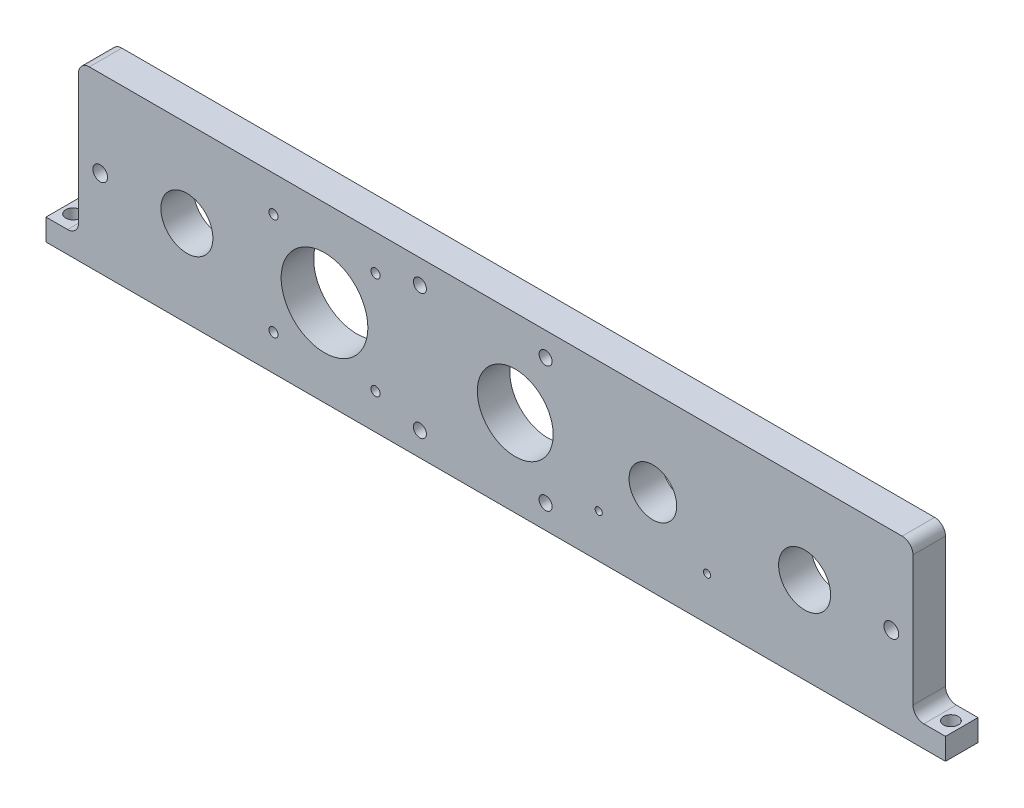
from build123d import *

# Parameters (mm, degrees)
BOSS_EXTRUDE1_DEPTH   = 7.5
SKETCH2_R             = 12
SKETCH2_R_2           = 17.5
SKETCH2_R_3           = 11
SKETCH2_R_4           = 20
SKETCH2_R_5           = 3.4
CUT_EXTRUDE1_DEPTH    = 15
SKETCH3_R             = 3
CUT_EXTRUDE2_DEPTH    = 15
SKETCH4_R             = 3.4
CUT_EXTRUDE3_DEPTH    = 223.514044501
FILLET1_R             = 5
M4_TAPPED_HOLE1_D     = 3.3
M5_TAPPED_HOLE1_D     = 4.2
SKETCH10_W            = 15
SKETCH10_H            = 40
CUT_EXTRUDE4_DEPTH    = 223.892911507
FILLET2_R             = 5
M6_TAPPED_HOLE1_D     = 5
M6_TAPPED_HOLE1_DEPTH = 15
M6_TAPPED_HOLE1_TIP   = 1.502151548


with BuildPart() as part:
    # Sketch1 → Boss-Extrude1 (new, symmetric)
    with BuildSketch(Plane.XY):
        Polygon((207.5, 0), (-207.5, 0), (-207.5, 10), (-192.5, 10), (-192.5, 70), (-207.5, 70), (-207.5, 80), (207.5, 80), (207.5, 70), (192.5, 70), (192.5, 10), (207.5, 10), align=None)
    extrude(amount=BOSS_EXTRUDE1_DEPTH, both=True)

    # Sketch2 → Cut-Extrude1 (cut)
    with BuildSketch(Plane.XY.offset(7.5)):
        with Locations((-142.5, 40)):
            Circle(SKETCH2_R)
        with Locations((9, 40)):
            Circle(SKETCH2_R_2)
        with Locations((72.5, 40)):
            Circle(SKETCH2_R_3)
        with Locations((-79, 40)):
            Circle(SKETCH2_R_4)
        with Locations((142.5, 40)):
            Circle(SKETCH2_R)
        with Locations((-182.5, 40)):
            Circle(SKETCH2_R_5)
        with Locations((182.5, 40)):
            Circle(SKETCH2_R_5)
    extrude(amount=-CUT_EXTRUDE1_DEPTH, mode=Mode.SUBTRACT)

    # Sketch3 → Cut-Extrude2 (cut)
    with BuildSketch(Plane.XY.offset(7.5)):
        with Locations((-35, 69)):
            Circle(SKETCH3_R)
        with Locations((23, 69)):
            Circle(SKETCH3_R)
        with Locations((23, 11)):
            Circle(SKETCH3_R)
        with Locations((-35, 11)):
            Circle(SKETCH3_R)
    extrude(amount=-CUT_EXTRUDE2_DEPTH, mode=Mode.SUBTRACT)

    # Sketch4 → Cut-Extrude3 (cut, through all)
    with BuildSketch(Plane(origin=(0, 80, 0), x_dir=(1, 0, 0), z_dir=(0, 1, 0))):
        with Locations(Location((-202.5, 0, 0), (0, 0, 270))):
            Circle(SKETCH4_R)
        with Locations(Location((202.5, 0, 0), (0, 0, 180))):
            Circle(SKETCH4_R)
    extrude(amount=-CUT_EXTRUDE3_DEPTH, mode=Mode.SUBTRACT)

    # Fillet1
    fillet1_edges = [part.edges().sort_by_distance(p)[0] for p in [
        (-192.5, 10, 0),
        (-192.5, 70, 0),
        (192.5, 70, 0),
        (192.5, 10, 0),
    ]]
    fillet(fillet1_edges, radius=FILLET1_R)

    # M4 Tapped Hole1 (through all)
    with Locations(Plane.XY.offset(7.5)):
        with Locations((47.5, 20), (97.5, 20)):
            Hole(M4_TAPPED_HOLE1_D / 2)

    # M5 Tapped Hole1 (through all)
    with Locations(Plane.XY.offset(7.5)):
        with Locations((-102.55, 63.55), (-55.45, 16.45), (-102.55, 16.45), (-55.45, 63.55)):
            Hole(M5_TAPPED_HOLE1_D / 2)

    # Sketch10 → Cut-Extrude4 (cut, through all)
    with BuildSketch(Plane.XY.offset(7.5)):
        with Locations((-200, 60)):
            Rectangle(SKETCH10_W, SKETCH10_H)
        with Locations((200, 60)):
            Rectangle(SKETCH10_W, SKETCH10_H)
    extrude(amount=-CUT_EXTRUDE4_DEPTH, mode=Mode.SUBTRACT)

    # Fillet2
    fillet2_edges = [part.edges().sort_by_distance(p)[0] for p in [
        (-192.5, 80, 0),
        (192.5, 80, 0),
    ]]
    fillet(fillet2_edges, radius=FILLET2_R)

    # M6 Tapped Hole1
    with Locations(Plane(origin=(0, 0, 0), x_dir=(-1, 0, 0), z_dir=(0, -1, 0))):
        with Locations((-125, 0), (125, 0)):
            Hole(M6_TAPPED_HOLE1_D / 2, depth=M6_TAPPED_HOLE1_DEPTH)
            with Locations((0, 0, -(M6_TAPPED_HOLE1_DEPTH + M6_TAPPED_HOLE1_TIP / 2))):  # 118° drill point
                Cone(0, M6_TAPPED_HOLE1_D / 2, M6_TAPPED_HOLE1_TIP, mode=Mode.SUBTRACT)


solid = part.part
